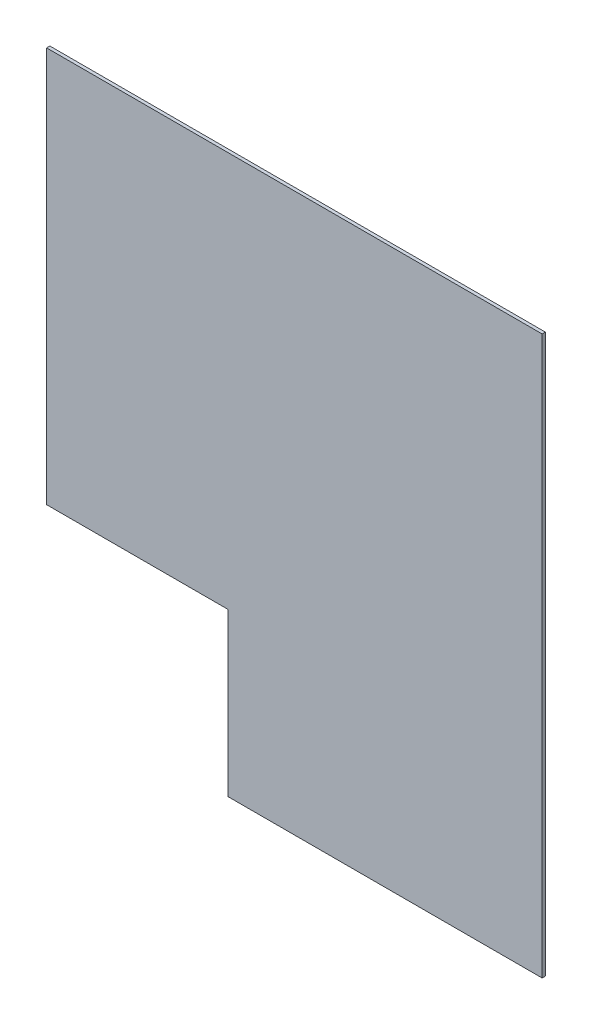
from build123d import *

# Parameters (mm, degrees)
SKETCH_1_W          = 764
SKETCH_1_H          = 860
EXTRUDE_1_DEPTH     = 5
CUT_EXTRUDE_1_REACH = 577.195
SKETCH_2_W          = 280
SKETCH_2_H          = 250


with BuildPart() as part:
    # 草图1 → 凸台-拉伸1 (new body)
    with BuildSketch(Plane.XY):
        Rectangle(SKETCH_1_W, SKETCH_1_H)
    extrude(amount=EXTRUDE_1_DEPTH)

    # 草图2 → 切除-拉伸1 (cut, up to next)
    with BuildSketch(Plane.XY.offset(5), mode=Mode.PRIVATE) as cut_extrude_1_sk1:
        with Locations((-242, -305)):
            Rectangle(SKETCH_2_W, SKETCH_2_H)
    cut_extrude_1_tool1 = extrude(cut_extrude_1_sk1.sketch, amount=-CUT_EXTRUDE_1_REACH, mode=Mode.PRIVATE) & part.part
    add(cut_extrude_1_tool1.solids().sort_by_distance((-242, -305, 5))[0], mode=Mode.SUBTRACT)


solid = part.part
